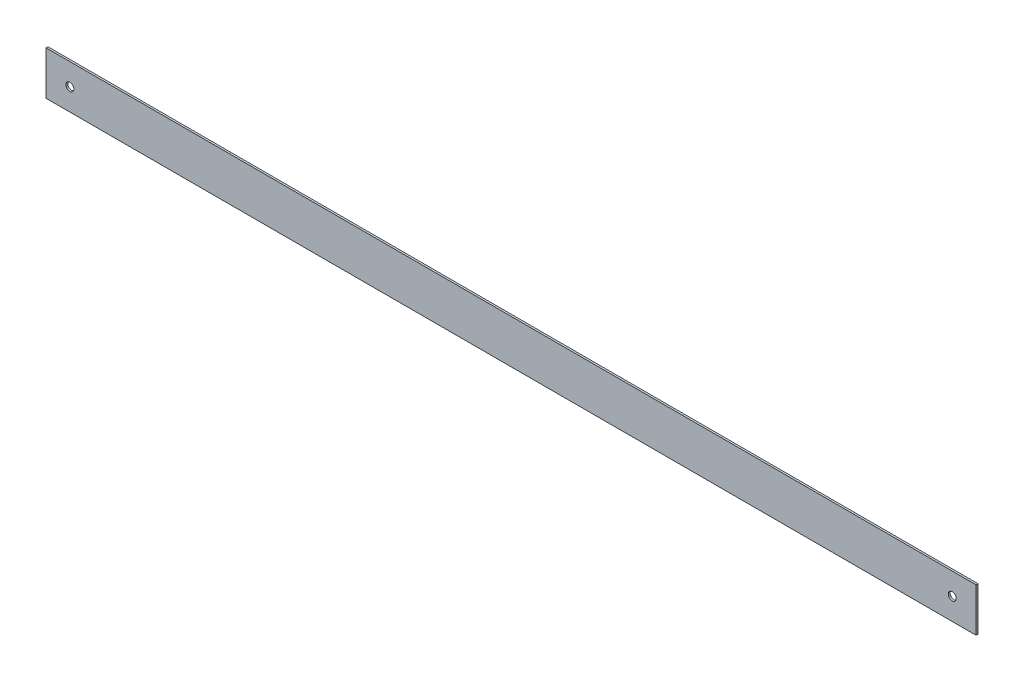
SolidWorks part; units mm, degrees
ref_plane "前视基准面" through (0, 0, 0) normal (0, 0, 1) x (1, 0, 0)
ref_plane "上视基准面" through (0, 0, 0) normal (0, 1, 0) x (1, 0, 0)
ref_plane "右视基准面" through (0, 0, 0) normal (1, 0, 0) x (0, 0, -1)
sketch "草图1" plane through (0, 0, 0) normal (0, 0, 1) x (1, 0, 0)
  line L1 (0, 0) -> (585, 0)
  line L2 (0, 0) -> (0, 27.5)
  line L3 (0, 27.5) -> (585, 27.5)
  line L4 (585, 0) -> (585, 27.5)
  dimension "D1" = 27.5
  dimension "D2" = 585
extrude "凸台-拉伸1" add sketch "草图1" along normal blind 1.2
hole_wizard "Ø5.0 (5) 直径孔1" positions "草图3" profile "草图2" hole size "Ø5.0" standard "GB"
sketch "草图3" plane through (0, 0, 1.2) normal (0, 0, 1) x (1, 0, 0)
  line L0 (0, 13.75) -> (35.4027, 13.75) construction
  line L1 (0, 27.5) -> (0, 0) construction
  line L3 (585, 13.75) -> (561.2006, 13.75) construction
  line L4 (585, 0) -> (585, 27.5) construction
  point P0 (15, 13.75)
  point P2 (570, 13.75)
  dimension "D1" = 15
  dimension "D2" = 15
sketch "草图2" plane through (15, 13.75, 1.2) normal (1, 0, 0) x (0, -1, 0)
  line L0 (0, 0) -> (0, 6.5022)
  line L1 (0, 6.5022) -> (2.5, 5)
  line L2 (2.5, 5) -> (2.5, 0)
  line L5 (2.5, 0) -> (0, 0)
  line L10 (0, 6.5022) -> (-2.5, 5) construction
  line L11 (0, -6.35) -> (0, 107.95) construction
  dimension "孔直径" = 5
  dimension "孔深度" = 5
  dimension "导头角度" = 118
